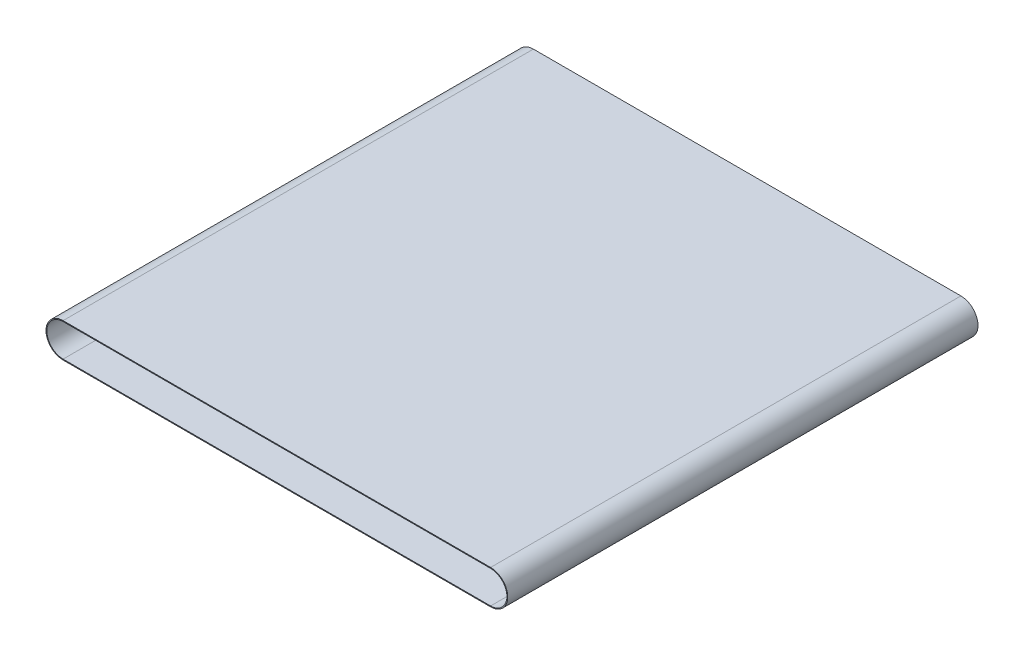
SolidWorks part; units mm, degrees
material "PVB"
ref_plane "前视基准面" through (0, 0, 0) normal (0, 0, 1) x (1, 0, 0)
ref_plane "上视基准面" through (0, 0, 0) normal (0, 1, 0) x (1, 0, 0)
ref_plane "右视基准面" through (0, 0, 0) normal (1, 0, 0) x (0, 0, -1)
sketch "草图1" plane through (0, 0, 0) normal (0, 0, 1) x (1, 0, 0)
  line L0 (-500, 0) -> (500, 0) construction
  line L1 (-500, 38) -> (500, 38)
  line L2 (-500, -38) -> (500, -38)
  arc A0 (-500, 38) -> (-500, -38) centre (-500, 0) ccw
  arc A1 (500, -38) -> (500, 38) centre (500, 0) ccw
  point P2 (0, 0)
  dimension "D1" = 76
  dimension "D2" = 1000
extrude "拉伸-薄壁1" add sketch "草图1" along normal mid plane 1100 thin thin type one direction wall 2
